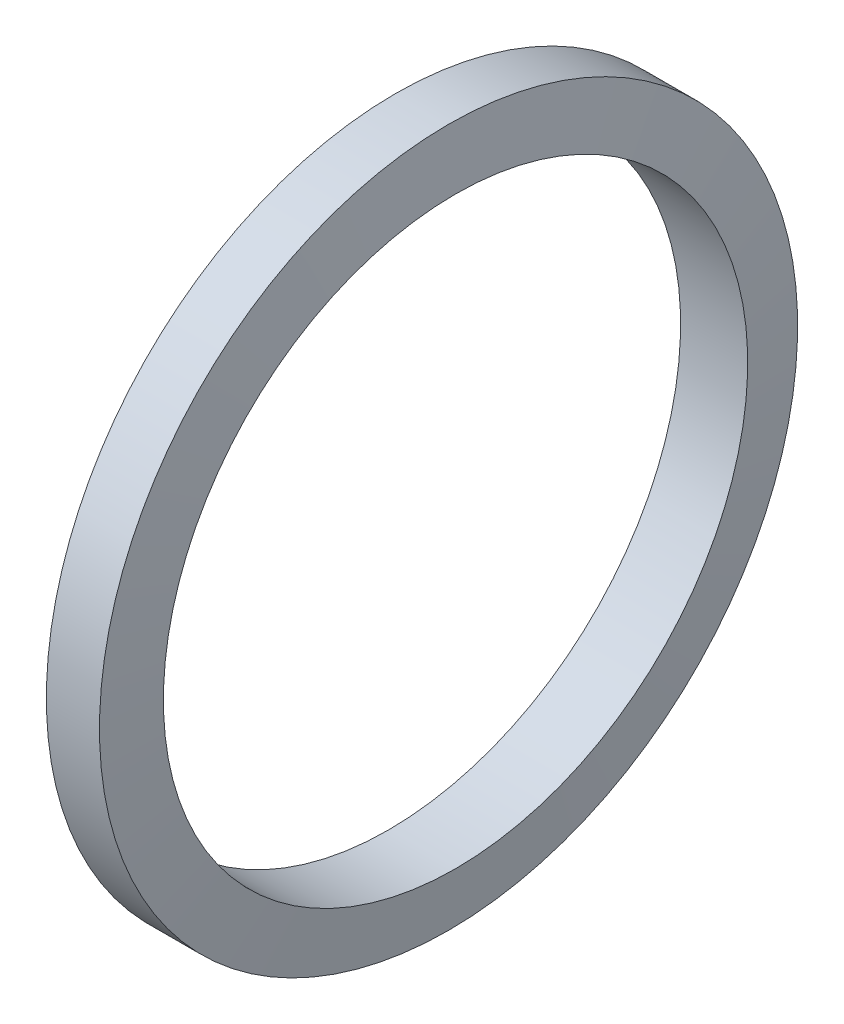
from build123d import *


with BuildPart() as part:
    # Sweep1: sweep along a path in Sketch3
    with BuildLine(Plane(origin=(0, 0, 0), x_dir=(0, 0, -1), z_dir=(1, 0, 0))) as sweep1_path:
        CenterArc((0, -46), 46, 0, 360)
    # Sketch2 → Sweep1 (sweep)
    with BuildSketch(Plane.XY):
        Polygon((-3.5, 0), (3.5, 0), (4.420884207, -7.5), (-4.420884207, -7.5), align=None)
    sweep(path=sweep1_path.line)


solid = part.part
